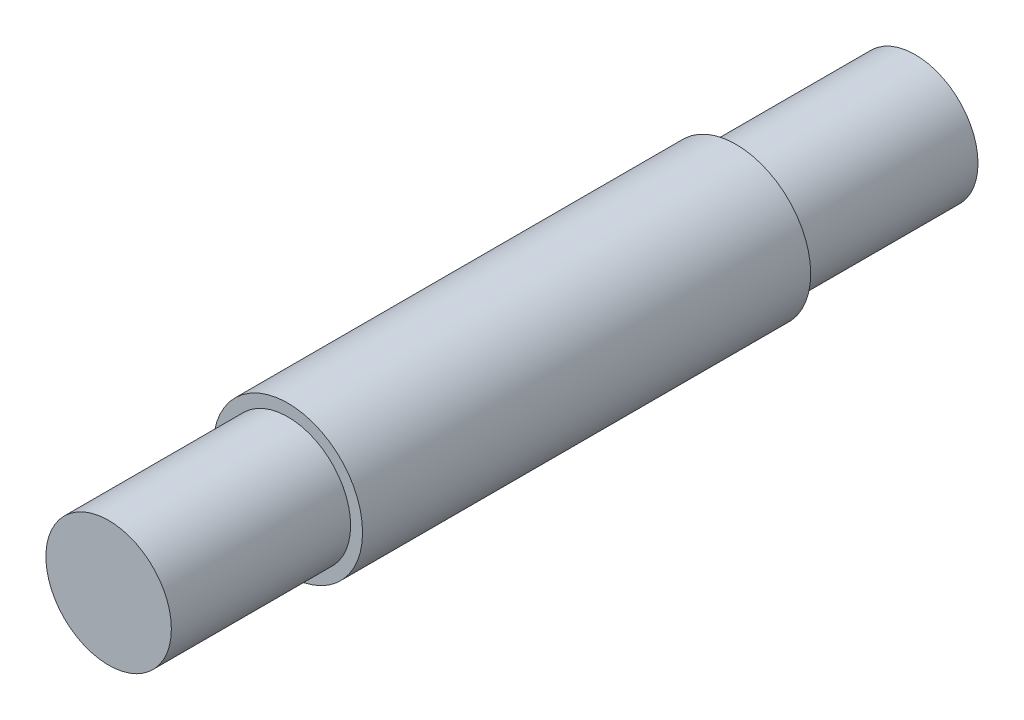
SolidWorks part; units mm, degrees
ref_plane "Front Plane" through (0, 0, 0) normal (0, 0, 1) x (1, 0, 0)
ref_plane "Top Plane" through (0, 0, 0) normal (0, 1, 0) x (1, 0, 0)
ref_plane "Right Plane" through (0, 0, 0) normal (1, 0, 0) x (0, 0, -1)
sketch "Sketch 1" plane through (0, 0, 0) normal (0, 0, 1) x (1, 0, 0)
  line L0 (0, 55.4084) -> (0, -50.1461) construction
  line L1 (-164.9606, 0) -> (173.305, 0) construction
  circle A0 centre (0, 0) radius 25
  dimension "D1" = 50
extrude "Boss-Extrude 1" add sketch "Sketch 1" along normal mid plane 150
sketch "Sketch 2" plane through (0, 0, 75) normal (0, 0, 1) x (1, 0, 0)
  circle A0 centre (0, 0) radius 21
  dimension "D1" = 42
extrude "Boss-Extrude 2" add sketch "Sketch 2" along normal blind 60
mirror "Mirror 1" about plane through (0, 0, 0) normal (0, 0, 1) of "Boss-Extrude 2"
